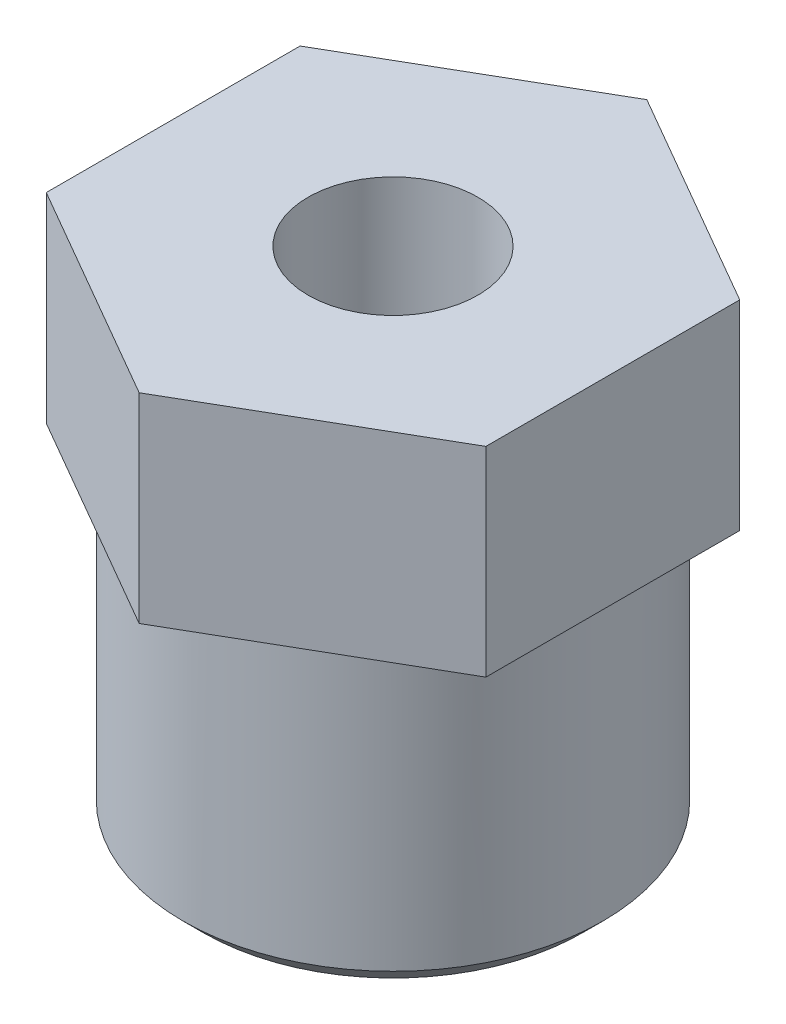
from build123d import *

# Parameters (mm, degrees)
BOSS_EXTRUDE1_DEPTH = 25
SKETCH3_OUTSIDE_W   = 32.376
SKETCH3_OUTSIDE_H   = 35.78
SKETCH3_OUTSIDE_R   = 10.5
CUT_EXTRUDE1_DEPTH  = 15
CHAMFER1_SIZE       = 1
M10_TAPPED_HOLE1_D  = 8.5


with BuildPart() as part:
    # Sketch1 → Boss-Extrude1 (new body)
    with BuildSketch(Plane(origin=(0, 0, 0), x_dir=(1, 0, 0), z_dir=(0, 1, 0))):
        Polygon((11, -6.350852961), (11, 6.350852961), (0, 12.701705922), (-11, 6.350852961), (-11, -6.350852961), (0, -12.701705922), align=None)
    extrude(amount=BOSS_EXTRUDE1_DEPTH)

    # Sketch3 outside → Cut-Extrude1 (cut)
    with BuildSketch(Plane.XZ):
        Rectangle(SKETCH3_OUTSIDE_W, SKETCH3_OUTSIDE_H)
        with Locations(Location((0, 0, 0), (0, 0, 270))):
            Circle(SKETCH3_OUTSIDE_R, mode=Mode.SUBTRACT)
    extrude(amount=-CUT_EXTRUDE1_DEPTH, mode=Mode.SUBTRACT)

    # Chamfer1
    chamfer1_edges = [part.edges().sort_by_distance(p)[0] for p in [
        (0, 0, 10.5),
    ]]
    chamfer(chamfer1_edges, length=CHAMFER1_SIZE)

    # M10 Tapped Hole1 (through all)
    with Locations(Plane.ZX.offset(25)):
        with Locations((0, 0)):
            Hole(M10_TAPPED_HOLE1_D / 2)


solid = part.part
